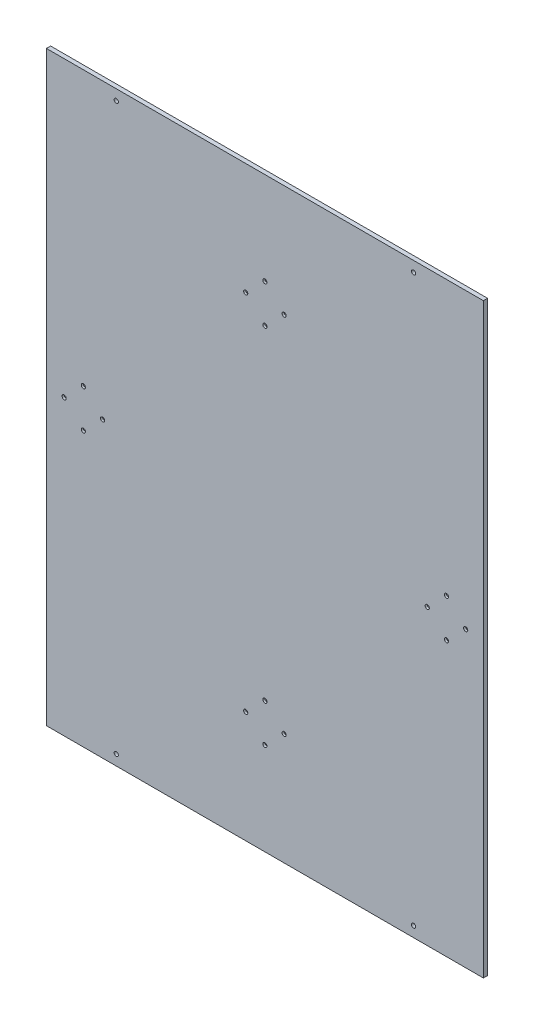
SolidWorks part; units mm, degrees
ref_plane "Front Plane" through (0, 0, 0) normal (0, 0, 1) x (1, 0, 0)
ref_plane "Top Plane" through (0, 0, 0) normal (0, 1, 0) x (1, 0, 0)
ref_plane "Right Plane" through (0, 0, 0) normal (1, 0, 0) x (0, 0, -1)
other "Configuration Table"
sketch "Sketch2" plane through (0, 0, 0) normal (0, 0, 1) x (1, 0, 0)
  line L1 (751.6646, 46.6218) -> (751.6646, -793.3782)
  line L2 (751.6646, -793.3782) -> (125.9792, -793.3782)
  line L3 (125.9792, -793.3782) -> (125.9792, 46.6218)
  line L4 (125.9792, 46.6218) -> (751.6646, 46.6218)
extrude "Boss-Extrude1" add sketch "Sketch2" along normal blind 6
sketch "Sketch3" plane through (0, 0, 6) normal (0, 0, 1) x (1, 0, 0)
  line L0 (438.8219, 46.6218) -> (438.8219, -373.3782) construction
  line L1 (751.6646, 46.6218) -> (125.9792, 46.6218) construction
  line L2 (125.9792, -373.3782) -> (438.8219, -373.3782) construction
  line L3 (125.9792, 46.6218) -> (125.9792, -793.3782) construction
  circle A5 centre (438.8219, -660.8782) radius 3
  circle A6 centre (411.3219, -633.3782) radius 3
  circle A7 centre (438.8219, -605.8782) radius 3
  circle A8 centre (466.3219, -633.3782) radius 3
  circle A9 centre (151.3219, -373.3782) radius 3
  circle A10 centre (178.8219, -345.8782) radius 3
  circle A11 centre (206.3219, -373.3782) radius 3
  circle A12 centre (178.8219, -400.8782) radius 3
  circle A13 centre (438.8219, -140.8782) radius 3
  circle A14 centre (411.3219, -113.3782) radius 3
  circle A15 centre (438.8219, -85.8782) radius 3
  circle A16 centre (466.3219, -113.3782) radius 3
  circle A17 centre (698.8219, -400.8782) radius 3
  circle A18 centre (671.3219, -373.3782) radius 3
  circle A19 centre (698.8219, -345.8782) radius 3
  circle A20 centre (726.3219, -373.3782) radius 3
  circle A21 centre (438.8219, -373.3782) radius 260
  point P21 (438.8219, -633.3782)
  point P30 (178.8219, -373.3782)
  point P39 (438.8219, -113.3782)
  point P48 (698.8219, -373.3782)
  dimension "D2" = 27.5
  dimension "D3" = 27.5
  dimension "D4" = 27.5
  dimension "D5" = 27.5
  dimension "D6" = 6
  dimension "D8" = 6
  dimension "D10" = 6
  dimension "D12" = 6
  dimension "D14" = 260
  dimension "D15" = 260
  dimension "D17" = 260
  dimension "D16" = 260
  dimension "D7" = 4
  dimension "D9" = 4
  dimension "D11" = 4
  dimension "D13" = 4
extrude "Cut-Extrude1" cut sketch "Sketch3" against normal blind 3 contours A6 | A7 | A8 | A5 | A10 | A11 | A12 | A9 | A13 | A14 | A16 | A15 | A18 | A17 | A20 | A19
sketch "Sketch6" plane through (0, 0, 6) normal (0, 0, 1) x (1, 0, 0)
  line L0 (125.9792, 46.6218) -> (125.9792, 31.6218)
  line L1 (125.9792, 46.6218) -> (125.9792, -793.3782) construction
  line L2 (125.9792, 31.6218) -> (751.6646, 31.6218)
  line L3 (751.6646, -793.3782) -> (751.6646, 46.6218) construction
  line L4 (751.6646, 31.6218) -> (651.6646, 31.6218)
  line L5 (125.9792, -793.3782) -> (125.9792, -778.3782)
  line L6 (125.9792, -778.3782) -> (751.6646, -778.3782)
  circle A0 centre (651.6646, 31.6218) radius 3
  circle A1 centre (225.9792, 31.6218) radius 3
  circle A2 centre (651.6646, -778.3782) radius 3
  circle A3 centre (225.9792, -778.3782) radius 3
  dimension "D1" = 6
  dimension "D2" = 6
  dimension "D4" = 6
  dimension "D6" = 6
  dimension "D3" = 100
  dimension "D5" = 100
  dimension "D7" = 100
  dimension "D8" = 100
extrude "Cut-Extrude2" cut sketch "Sketch6" against normal blind 36 contours L6 A2 | L6 A2 | L6 A3 | L6 A3 | L2 A1 | L2 A1 | L2 A0 | L2 A0
